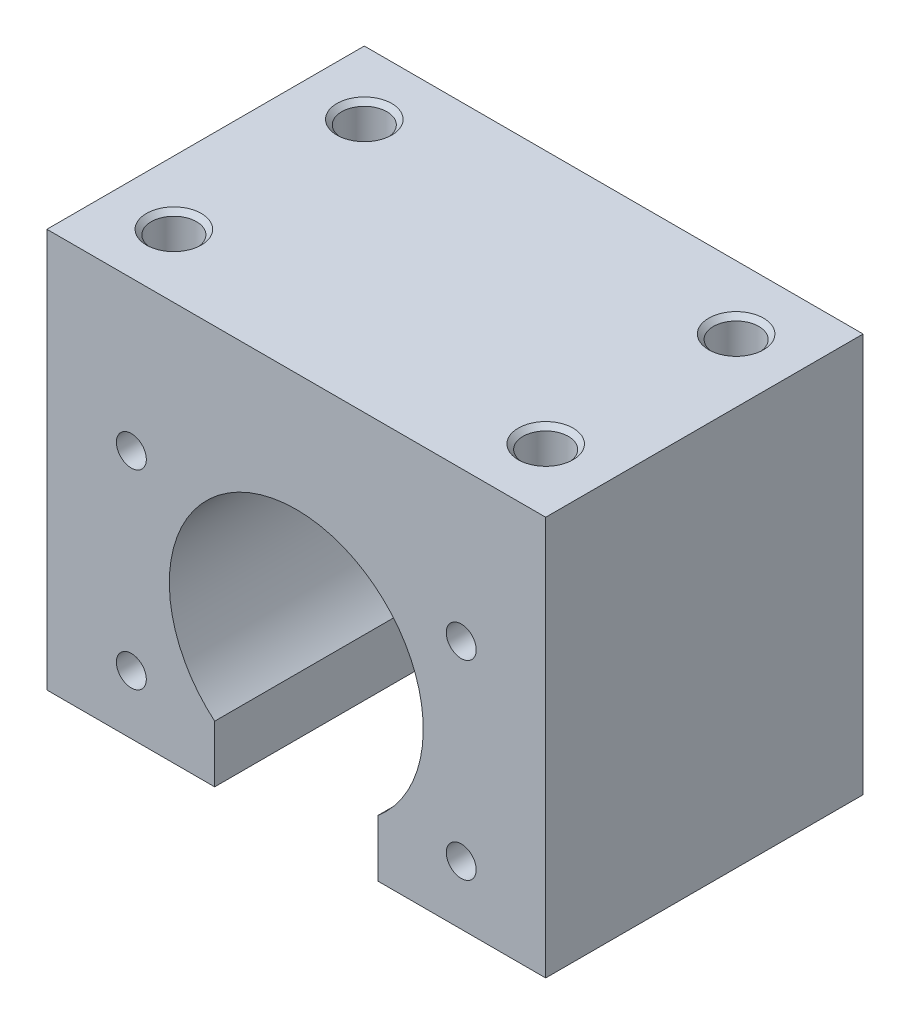
from build123d import *

# Parameters (mm, degrees)
EXTRUDE_1_DEPTH              = 17.5
HOLE_WIZARD_M4_1_D           = 3.3
HOLE_WIZARD_M4_1_DEPTH       = 9.5
HOLE_WIZARD_M4_1_TIP         = 0.991420021
HOLE_WIZARD_M6_1_D           = 5
HOLE_WIZARD_M6_1_DEPTH       = 12
HOLE_WIZARD_M6_1_CSINK_D     = 6.05
HOLE_WIZARD_M6_1_CSINK_ANGLE = 90
HOLE_WIZARD_M6_1_TIP         = 1.502151548


with BuildPart() as part:
    # 草图1 → 凸台-拉伸1 (new, symmetric)
    with BuildSketch(Plane.XY):
        with BuildLine():
            Line((-27.5, 27), (27.5, 27))
            Line((27.5, 27), (27.5, -17))
            Line((27.5, -17), (9, -17))
            Line((9, -17), (9, -10.723805295))
            ThreePointArc((9, -10.723805295), (0, 14), (-9, -10.723805295))
            Line((-9, -10.723805295), (-9, -17))
            Line((-9, -17), (-27.5, -17))
            Line((-27.5, -17), (-27.5, 27))
        make_face()
    extrude(amount=EXTRUDE_1_DEPTH, both=True)

    # M4 螺纹孔1
    with Locations(Plane.XY.offset(17.5)):
        with Locations((18.186533479, 10.5), (18.186533479, -10.5), (-18.186533479, -10.5), (-18.186533479, 10.5)):
            Hole(HOLE_WIZARD_M4_1_D / 2, depth=HOLE_WIZARD_M4_1_DEPTH)
            with Locations((0, 0, -(HOLE_WIZARD_M4_1_DEPTH + HOLE_WIZARD_M4_1_TIP / 2))):  # 118° drill point
                Cone(0, HOLE_WIZARD_M4_1_D / 2, HOLE_WIZARD_M4_1_TIP, mode=Mode.SUBTRACT)

    # M6 螺纹孔1
    with Locations(Plane(origin=(-20.5, 27, 10.5), x_dir=(0, 0, 1), z_dir=(0, 1, 0))):
        with Locations((0, 0), (-21, 0), (-21, 41), (0, 41)):
            CounterSinkHole(HOLE_WIZARD_M6_1_D / 2, HOLE_WIZARD_M6_1_CSINK_D / 2, depth=HOLE_WIZARD_M6_1_DEPTH, counter_sink_angle=HOLE_WIZARD_M6_1_CSINK_ANGLE)
            with Locations((0, 0, -(HOLE_WIZARD_M6_1_DEPTH + HOLE_WIZARD_M6_1_TIP / 2))):  # 118° drill point
                Cone(0, HOLE_WIZARD_M6_1_D / 2, HOLE_WIZARD_M6_1_TIP, mode=Mode.SUBTRACT)


solid = part.part
